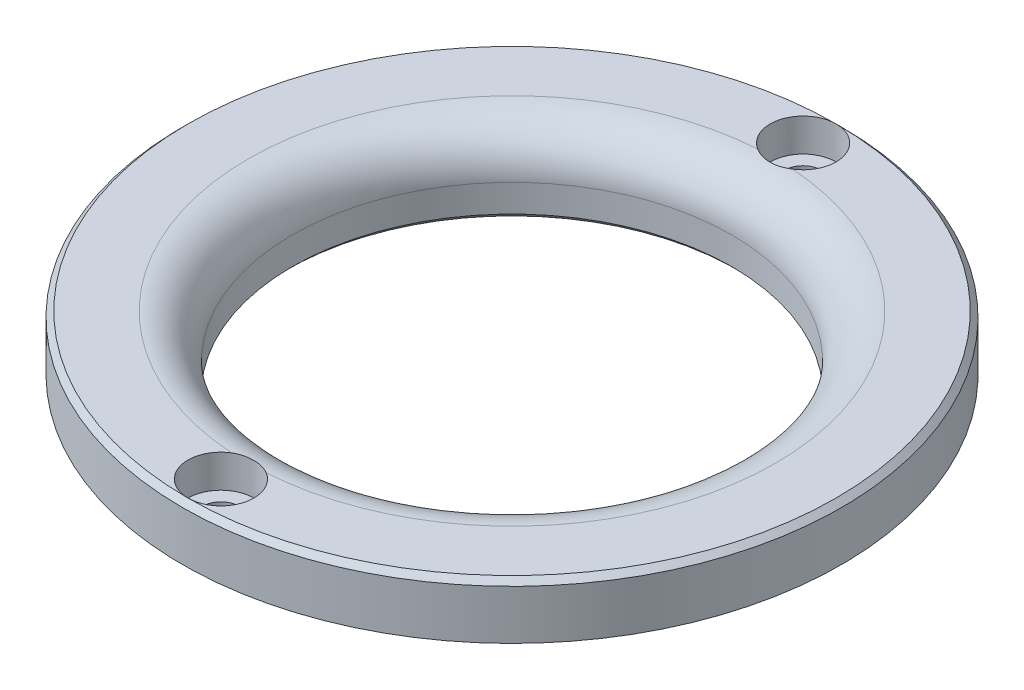
SolidWorks part; units mm, degrees
ref_plane "前视" through (0, 0, 0) normal (0, 0, 1) x (1, 0, 0)
ref_plane "上视" through (0, 0, 0) normal (0, 1, 0) x (1, 0, 0)
ref_plane "右视" through (0, 0, 0) normal (1, 0, 0) x (0, 0, -1)
sketch "草图1" plane through (0, 0, 0) normal (0, 1, 0) x (1, 0, 0)
  circle A0 centre (0, 0) radius 20
  circle A1 centre (0, 0) radius 30
  dimension "D1" = 40
  dimension "D2" = 60
extrude "凸台-拉伸1" add sketch "草图1" along normal mid plane 7
sketch "草图2" plane through (0, -3.5, 0) normal (0, -1, 0) x (1, 0, 0)
  circle A0 centre (0, 0) radius 23
  dimension "D1" = 46
extrude "切除-拉伸1" cut sketch "草图2" against normal blind 2 flip side to cut
fillet "圆角1" radius 4 1 edges at (0, 3.5, 20)
chamfer "倒角1" distance 0.5 angle 45 3 edges at (0, -3.5, -23) (0, -3.5, 20) (0, 3.5, 30)
hole_wizard "打孔尺寸根据内六角圆柱头螺钉的类型1" positions "草图4" profile "草图3" counterbore size "M3" standard "Gb" end condition through all
sketch "草图4" plane through (0, 3.5, 0) normal (0, 1, 0) x (1, 0, 0)
  line L0 (0, 0) -> (42.9503, 0) construction
  point P0 (0, -26.5)
  point P2 (0, 26.5)
  dimension "D1" = 53
sketch "草图3" plane through (0, 3.5, 26.5) normal (1, 0, 0) x (0, 0, 1)
  line L0 (0, 0) -> (0, 7)
  line L1 (0, 7) -> (1.7, 7)
  line L3 (1.7, 7) -> (1.7, 3)
  line L4 (1.7, 3) -> (3, 3)
  line L5 (3, 3) -> (3, 0)
  line L7 (3, 0) -> (0, 0)
  line L11 (0, -6.35) -> (0, 107.95) construction
  dimension "通孔孔直径" = 3.4
  dimension "通孔孔深度" = 7
  dimension "柱形沉头孔直径" = 6
  dimension "柱形沉头孔深度" = 3
